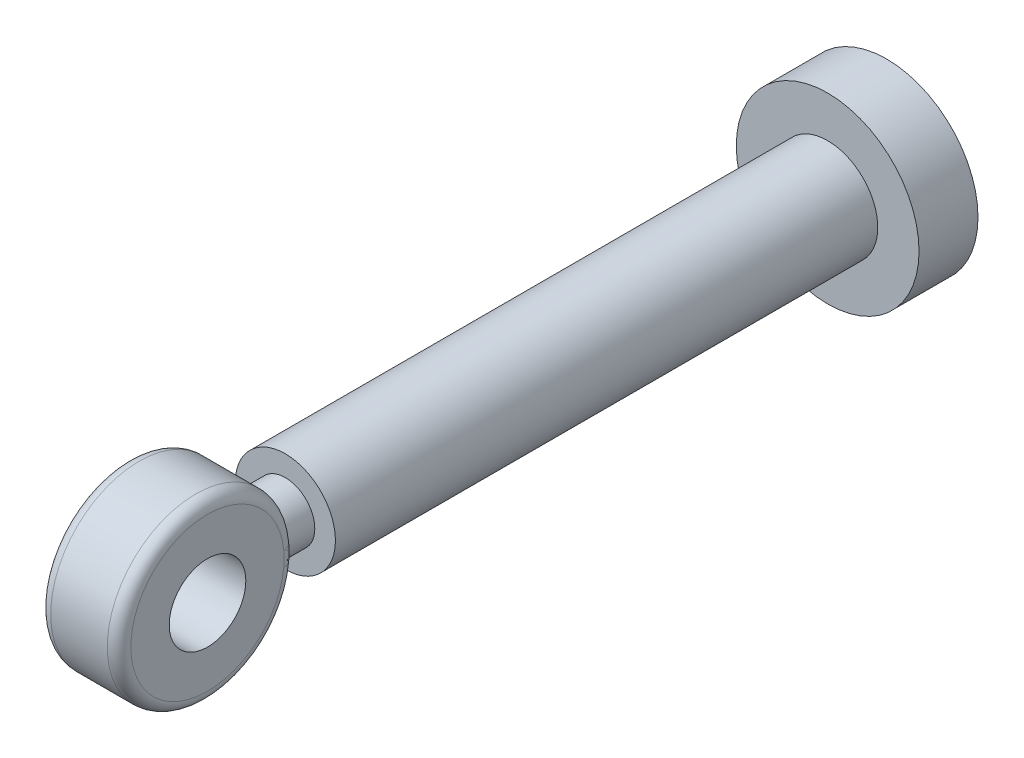
SolidWorks part; units mm, degrees
material "1.0503 (C45)"
ref_plane "前视基准面" through (0, 0, 0) normal (0, 0, 1) x (1, 0, 0)
ref_plane "上视基准面" through (0, 0, 0) normal (0, 1, 0) x (1, 0, 0)
ref_plane "右视基准面" through (0, 0, 0) normal (1, 0, 0) x (0, 0, -1)
sketch "草图1" plane through (0, 0, 0) normal (0, 0, 1) x (1, 0, 0)
  circle A0 centre (0, 0) radius 42.5
  dimension "D1" = 85
extrude "凸台-拉伸1" add sketch "草图1" along normal blind 460
sketch "草图2" plane through (0, 0, 0) normal (0, 0, -1) x (-1, 0, 0)
  circle A0 centre (0, 0) radius 77.5
  dimension "D1" = 155
extrude "凸台-拉伸2" add sketch "草图2" along normal blind 50
sketch "草图3" plane through (0, 0, 0) normal (1, 0, 0) x (0, 0, -1)
  line L0 (-460, 0) -> (-560, 0) construction
  line L1 (-460, 42.5) -> (-460, -42.5) construction
  line L2 (85.25, 0) -> (-85.25, 0) construction
  circle A0 centre (-560, 0) radius 32.5
  circle A1 centre (-560, 0) radius 75
  dimension "D1" = 65
  dimension "D2" = 150
  dimension "D3" = 100
extrude "凸台-拉伸3" add sketch "草图3" along normal mid plane 68 separate body
sketch "草图4" plane through (0, 0, 460) normal (0, 0, 1) x (1, 0, 0)
  circle A0 centre (0, 0) radius 25
extrude "凸台-拉伸4" add sketch "草图4" along normal up to surface (25 mm away) up to face at (34, 0, 485)
fillet "圆角1" radius 10 2 edges at (-34, 0, 485) (34, 0, 485)
sketch "草图5" plane through (0, 0, 0) normal (0, 1, 0) x (1, 0, 0)
  line L0 (0, -527.5) -> (0, -592.5) construction
  line L1 (34, -527.5) -> (-34, -527.5) construction
  line L2 (-34, -592.5) -> (34, -592.5) construction
  line L3 (0, -510) -> (0, -610)
  arc A0 (0, -610) -> (0, -510) centre (0, -560) ccw
  dimension "D1" = 100
revolve "切除-旋转3" [suppressed] cut sketch "草图5" angle 360 about L0
